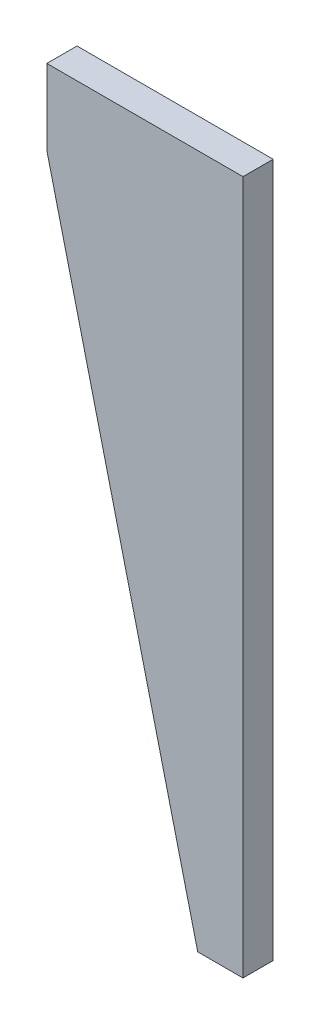
from build123d import *

# Parameters (mm, degrees)
SKETCH1_W           = 130
SKETCH1_H           = 460
BOSS_EXTRUDE1_DEPTH = 10
CUT_EXTRUDE1_DEPTH  = 240.843699104


with BuildPart() as part:
    # Sketch1 → Boss-Extrude1 (new, symmetric)
    with BuildSketch(Plane.XY):
        Rectangle(SKETCH1_W, SKETCH1_H)
    extrude(amount=BOSS_EXTRUDE1_DEPTH, both=True)

    # Sketch2 → Cut-Extrude1 (cut, through all)
    with BuildSketch(Plane.XY.offset(10)):
        Polygon((-65, 180), (35, -230), (-65, -230), align=None)
    extrude(amount=-CUT_EXTRUDE1_DEPTH, mode=Mode.SUBTRACT)


solid = part.part
